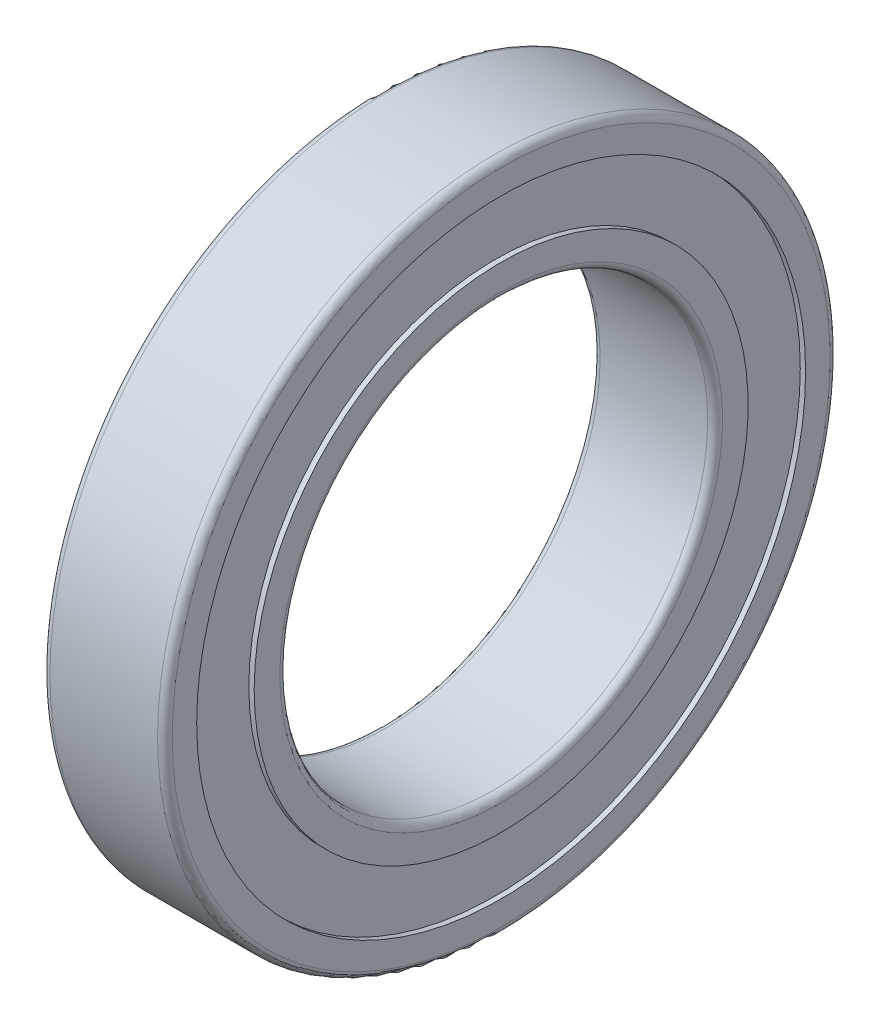
SolidWorks part; units mm, degrees
ref_plane "Front Plane" through (0, 0, 0) normal (0, 0, 1) x (1, 0, 0)
ref_plane "Top Plane" through (0, 0, 0) normal (0, 1, 0) x (1, 0, 0)
ref_plane "Right Plane" through (0, 0, 0) normal (1, 0, 0) x (0, 0, -1)
sketch "Sketch1" plane through (0, 0, 0) normal (0, 0, 1) x (1, 0, 0)
  line L0 (0, 0) -> (10, 0) construction
  line L1 (0, 17.5) -> (10, 17.5)
  line L2 (0, 27.5) -> (10, 27.5)
  line L3 (0, 27.5) -> (0, 24.9)
  line L4 (0, 24.9) -> (0.435, 24.9)
  line L5 (10, 27.5) -> (10, 24.9)
  line L6 (0.435, 24.9) -> (0.435, 20.2)
  line L7 (0.435, 20.2) -> (0, 20.2)
  line L8 (0, 20.2) -> (0, 17.5)
  line L9 (10, 24.9) -> (9.565, 24.9)
  line L10 (9.565, 24.9) -> (9.565, 20.2)
  line L11 (9.565, 20.2) -> (10, 20.2)
  line L12 (10, 20.2) -> (10, 17.5)
  dimension "D" = 55
  dimension "B" = 10
  dimension "D_s" = 35
  dimension "MSM_1" = 49.8
  dimension "MSM_2" = 40.4
  dimension "MSM_3" = 0.435
revolve "Revolve1" add sketch "Sketch1" angle 360 about L0
fillet "Fillet1" radius 0.6 2 edges at (10, 0, 27.5) (0, 0, 27.5)
fillet "Fillet2" radius 0.6 2 edges at (10, 0, 17.5) (0, 0, 17.5)
